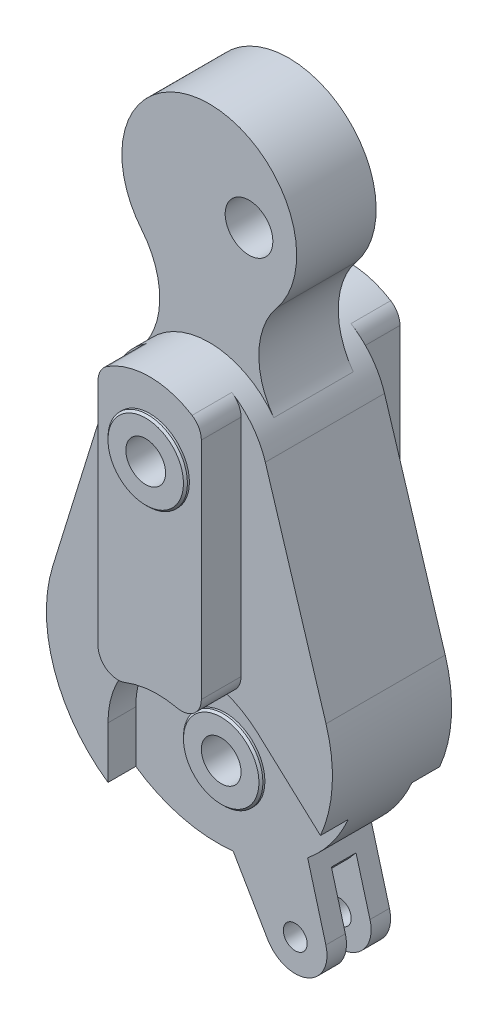
from build123d import *

# Parameters (mm, degrees)
SKETCH_1_3_R             = 6
BOSS_EXTRUDE1_DEPTH      = 10
BOSS_EXTRUDE2_DEPTH      = 15
BOSS_EXTRUDE3_START      = 10
BOSS_EXTRUDE3_DEPTH      = 10
CUT_EXTRUDE1_DEPTH       = 7
SKETCH4_R                = 10
BOSS_EXTRUDE4_DEPTH      = 1
CHAMFER1_SIZE            = 0.5
SKETCH5_R                = 10
BOSS_EXTRUDE5_DEPTH      = 1
CHAMFER2_SIZE            = 0.5
CHAMFER1_OF_MIRROR2_SIZE = 0.5
CHAMFER2_OF_MIRROR2_SIZE = 0.5
SKETCH6_R                = 5
CUT_EXTRUDE3_DEPTH       = 90
BOSS_EXTRUDE7_DEPTH      = 8
CUT_EXTRUDE4_DEPTH       = 3.1
SKETCH8_R                = 3
CUT_EXTRUDE5_DEPTH       = 26.1


with BuildPart() as part:
    # Sketch 1_3 → Boss-Extrude1 (new, symmetric)
    with BuildSketch(Plane.XY):
        with BuildLine():
            ThreePointArc((-17.008171865, -13.954285714), (-12.480205961, -26.005740026), (-16.235073144, -38.32))
            ThreePointArc((-16.235073144, -38.32), (0, -30), (16.235073144, -38.32))
            ThreePointArc((16.235073144, -38.32), (12.480205961, -26.005740026), (17.008171865, -13.954285714))
            ThreePointArc((17.008171865, -13.954285714), (0, 22), (-17.008171865, -13.954285714))
        make_face()
        with Locations((10, 0)):
            Circle(SKETCH_1_3_R, mode=Mode.SUBTRACT)
    extrude(amount=BOSS_EXTRUDE1_DEPTH, both=True)

    # Sketch 1_3 2 → Boss-Extrude2 (add, symmetric)
    with BuildSketch(Plane.XY):
        with BuildLine():
            Line((-19.105316093, -44.085027726), (-34.389568967, -93.453049908))
            ThreePointArc((-34.389568967, -93.453049908), (0, -140.1), (34.389568967, -93.453049908))
            Line((34.389568967, -93.453049908), (19.105316093, -44.085027726))
            ThreePointArc((19.105316093, -44.085027726), (0, -30), (-19.105316093, -44.085027726))
        make_face()
    extrude(amount=BOSS_EXTRUDE2_DEPTH, both=True)

    # Sketch 3_4 → Boss-Extrude3 (add)
    with BuildSketch(Plane.XY.offset(15).offset(BOSS_EXTRUDE3_START)):
        with BuildLine():
            ThreePointArc((-10.666666667, -33.081896613), (-12.377975179, -34.896193002), (-13, -37.31142246))
            Line((-13, -37.31142246), (-13, -95.082623085))
            ThreePointArc((-13, -95.082623085), (-10.820380374, -99.211237204), (-6.181818182, -99.740327979))
            ThreePointArc((-6.181818182, -99.740327979), (0.289205667, -98.265134662), (6.909090909, -98.74206689))
            ThreePointArc((6.909090909, -98.74206689), (11.126136157, -97.764740023), (13, -93.862526199))
            Line((13, -93.862526199), (13, -37.31142246))
            ThreePointArc((13, -37.31142246), (12.377975179, -34.896193002), (10.666666667, -33.081896613))
            ThreePointArc((10.666666667, -33.081896613), (0, -30), (-10.666666667, -33.081896613))
        make_face()
    boss_extrude3 = extrude(amount=-BOSS_EXTRUDE3_DEPTH)

    # Sketch 3_4 2 → Cut-Extrude1 (cut)
    with BuildSketch(Plane.XY.offset(15)):
        with BuildLine():
            ThreePointArc((6.909090909, -98.74206689), (0.289205667, -98.265134662), (-6.181818182, -99.740327979))
            ThreePointArc((-6.181818182, -99.740327979), (-16.578763537, -108.008288317), (-20.5, -120.7))
            Line((-20.5, -120.7), (-20.5, -133.693073514))
            ThreePointArc((-20.5, -133.693073514), (9.82308926, -138.733898386), (32.984269817, -118.523520535))
            Line((32.984269817, -118.523520535), (17.171803721, -104.084754836))
            ThreePointArc((17.171803721, -104.084754836), (12.38973825, -100.742461597), (6.909090909, -98.74206689))
        make_face()
    cut_extrude1 = extrude(amount=-CUT_EXTRUDE1_DEPTH, mode=Mode.SUBTRACT)

    # Mirror1: Boss-Extrude3, Cut-Extrude1 across plane
    add(boss_extrude3.mirror(Plane.XY))
    add(cut_extrude1.mirror(Plane.XY), mode=Mode.SUBTRACT)

    # Sketch4 → Boss-Extrude4 (add)
    with BuildSketch(Plane.XY.offset(25)):
        with Locations((0, -48)):
            Circle(SKETCH4_R)
    boss_extrude4 = extrude(amount=BOSS_EXTRUDE4_DEPTH)

    # Chamfer1
    chamfer1_edges = [part.edges().sort_by_distance(p)[0] for p in [
        (-10, -48, 26),
    ]]
    chamfer(chamfer1_edges, length=CHAMFER1_SIZE)

    # Sketch5 → Boss-Extrude5 (add)
    with BuildSketch(Plane.XY.offset(8)):
        with Locations((2, -120.7)):
            Circle(SKETCH5_R)
    boss_extrude5 = extrude(amount=BOSS_EXTRUDE5_DEPTH)

    # Chamfer2
    chamfer2_edges = [part.edges().sort_by_distance(p)[0] for p in [
        (-8, -120.7, 9),
    ]]
    chamfer(chamfer2_edges, length=CHAMFER2_SIZE)

    # Mirror2: Boss-Extrude4, Boss-Extrude5 across plane
    add(boss_extrude4.mirror(Plane.XY))
    add(boss_extrude5.mirror(Plane.XY))

    # Chamfer1 of Mirror2
    chamfer1_of_mirror2_edges = [part.edges().sort_by_distance(p)[0] for p in [
        (-10, -48, -26),
    ]]
    chamfer(chamfer1_of_mirror2_edges, length=CHAMFER1_OF_MIRROR2_SIZE)

    # Chamfer2 of Mirror2
    chamfer2_of_mirror2_edges = [part.edges().sort_by_distance(p)[0] for p in [
        (-8, -120.7, -9),
    ]]
    chamfer(chamfer2_of_mirror2_edges, length=CHAMFER2_OF_MIRROR2_SIZE)

    # Sketch6 → Cut-Extrude3 (cut)
    with BuildSketch(Plane.XY.offset(26)):
        with Locations((0, -48)):
            Circle(SKETCH6_R)
        with Locations((2, -120.7)):
            Circle(SKETCH6_R)
    extrude(amount=-CUT_EXTRUDE3_DEPTH, mode=Mode.SUBTRACT)

    # Sketch 7_4 → Boss-Extrude7 (add, symmetric)
    with BuildSketch(Plane.XY):
        with BuildLine():
            ThreePointArc((7.265439801, -145.485820602), (16.504414385, -142.348085848), (23.838635926, -135.912775046))
            Line((23.838635926, -135.912775046), (22.762040961, -131.990670327))
            ThreePointArc((22.762040961, -131.990670327), (13.94801059, -137.288145483), (3.995857269, -139.877550569))
            Line((3.995857269, -139.877550569), (7.265439801, -145.485820602))
        make_face()
        with BuildLine():
            ThreePointArc((12.722682919, -154.846554807), (22.733495344, -158.1924848), (27.348577363, -148.699717507))
            Line((27.348577363, -148.699717507), (23.838635926, -135.912775046))
            ThreePointArc((23.838635926, -135.912775046), (16.504414385, -142.348085848), (7.265439801, -145.485820602))
            Line((7.265439801, -145.485820602), (12.722682919, -154.846554807))
        make_face()
    extrude(amount=BOSS_EXTRUDE7_DEPTH, both=True)

    # Sketch 7_4 2 → Cut-Extrude4 (cut, symmetric)
    with BuildSketch(Plane.XY):
        with BuildLine():
            ThreePointArc((12.722682919, -154.846554807), (22.733495344, -158.1924848), (27.348577363, -148.699717507))
            Line((27.348577363, -148.699717507), (23.838635926, -135.912775046))
            ThreePointArc((23.838635926, -135.912775046), (16.504414385, -142.348085848), (7.265439801, -145.485820602))
            Line((7.265439801, -145.485820602), (12.722682919, -154.846554807))
        make_face()
    extrude(amount=CUT_EXTRUDE4_DEPTH, both=True, mode=Mode.SUBTRACT)

    # Sketch8 → Cut-Extrude5 (cut, symmetric)
    with BuildSketch(Plane.XY.offset(8)):
        with Locations((19.633937435, -150.817341359)):
            Circle(SKETCH8_R)
    extrude(amount=CUT_EXTRUDE5_DEPTH, both=True, mode=Mode.SUBTRACT)


solid = part.part
